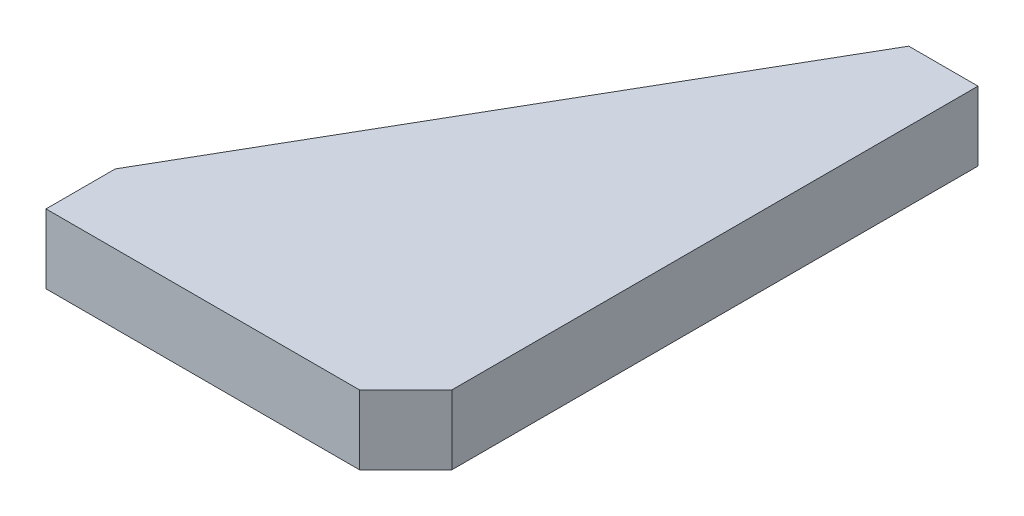
from build123d import *

# Parameters (mm, degrees)
EXTRUDE_1_DEPTH = 30


with BuildPart() as part:
    # 草图1 → 凸台-拉伸1 (new body)
    with BuildSketch(Plane(origin=(0, 0, 0), x_dir=(1, 0, 0), z_dir=(0, 1, 0))):
        Polygon((0, 0), (0, -228), (-20, -248), (-155.862358683, -248), (-155.862358683, -218), (-30, 0), align=None)
    extrude(amount=EXTRUDE_1_DEPTH)


solid = part.part
